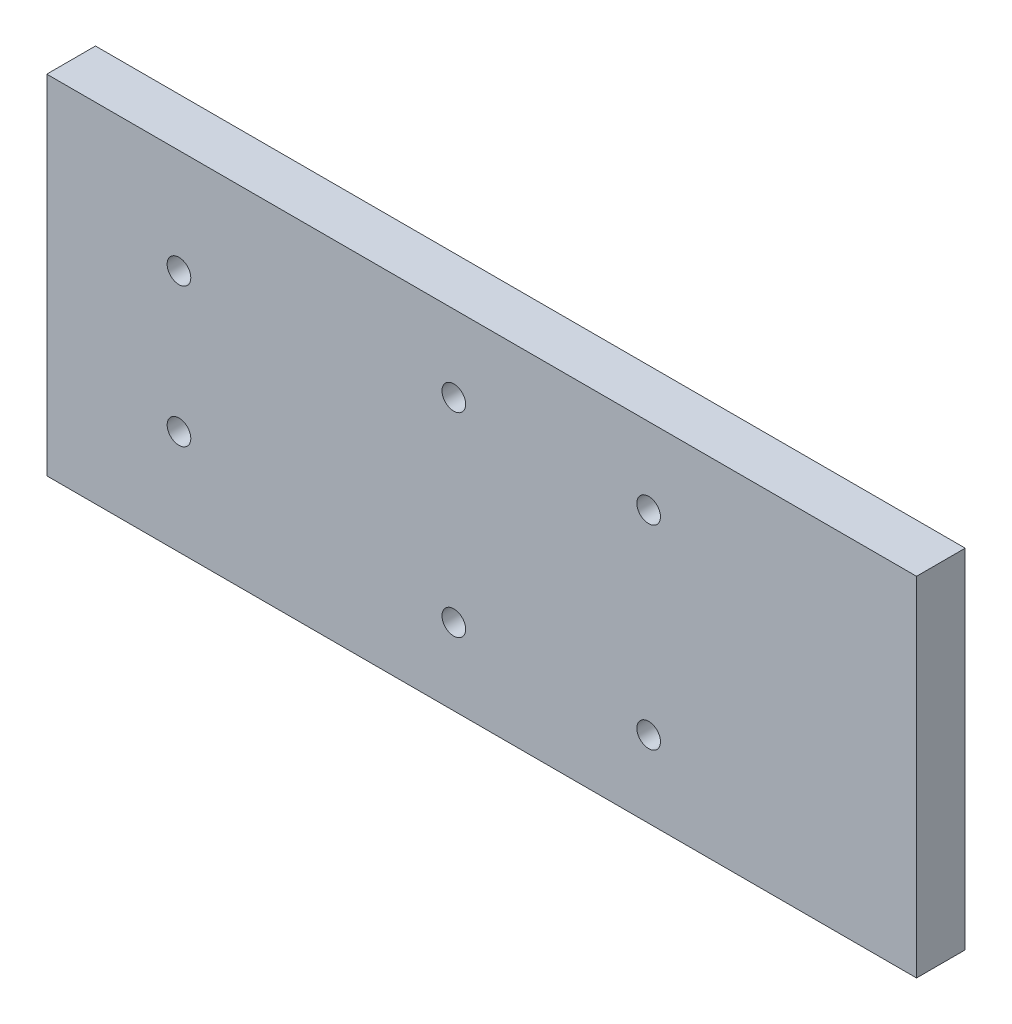
SolidWorks part; units mm, degrees
material "普通碳钢"
ref_plane "Front Plane" through (0, 0, 0) normal (0, 0, 1) x (1, 0, 0)
ref_plane "Top Plane" through (0, 0, 0) normal (0, 1, 0) x (1, 0, 0)
ref_plane "Right Plane" through (0, 0, 0) normal (1, 0, 0) x (0, 0, -1)
sketch "Sketch1" plane through (0, 0, 0) normal (0, 0, 1) x (1, 0, 0)
  line L0 (0, 50) -> (250, 50) construction
  line L1 (0, 0) -> (250, 0)
  line L2 (0, 0) -> (0, 100)
  line L3 (0, 100) -> (250, 100)
  line L4 (250, 0) -> (250, 100)
  line L6 (145, 100) -> (145, 0) construction
  circle A0 centre (117, 78) radius 2.5
  circle A1 centre (173, 78) radius 2.5
  circle A2 centre (117, 22) radius 2.5
  circle A3 centre (173, 22) radius 2.5
  dimension "D4" = 5
  dimension "D1" = 100
  dimension "D2" = 250
  dimension "D3" = 105
  dimension "D5" = 28
  dimension "D6" = 56
  dimension "D7" = 56
  dimension "D8" = 28
extrude "Boss-Extrude1" add sketch "Sketch1" along normal blind 14
hole_wizard "M8 Tapped Hole1" positions "Sketch2" profile "Sketch3" tap size "M8" standard "GB"
sketch "Sketch2" plane through (0, 0, 14) normal (0, 0, 1) x (1, 0, 0)
  point P0 (117, 78)
  point P3 (173, 78)
  point P6 (117, 22)
  point P9 (173, 22)
sketch "Sketch3" plane through (117, 78, 14) normal (1, 0, 0) x (0, -1, 0)
  line L0 (0, 0) -> (0, 21.7929)
  line L1 (0, 21.7929) -> (3.4, 19.75)
  line L2 (3.4, 19.75) -> (3.4, 0)
  line L5 (3.4, 0) -> (0, 0)
  line L10 (0, 21.7929) -> (-3.4, 19.75) construction
  line L11 (0, -6.35) -> (0, 107.95) construction
  dimension "螺纹孔钻头直径" = 6.8
  dimension "螺纹孔钻头深度" = 19.75
  dimension "导头角度" = 118
cosmetic thread "Cosmetic Thread1" parameters "D1"=14, "D2"=8
cosmetic thread "Cosmetic Thread2" parameters "D1"=14, "D2"=8
cosmetic thread "Cosmetic Thread3" parameters "D1"=14, "D2"=8
cosmetic thread "Cosmetic Thread4" parameters "D1"=14, "D2"=8
hole_wizard "M8 Tapped Hole2" positions "Sketch4" profile "Sketch5" tap size "M8" standard "GB" end condition through all
sketch "Sketch4" plane through (0, 0, 14) normal (0, 0, 1) x (1, 0, 0)
  line L0 (0, 50) -> (6.9633, 50) construction
  line L1 (0, 100) -> (0, 0) construction
  point P0 (38, 70)
  point P2 (38, 30)
  dimension "D1" = 40
  dimension "D2" = 38
sketch "Sketch5" plane through (38, 70, 14) normal (1, 0, 0) x (0, -1, 0)
  line L0 (0, 0) -> (0, 14)
  line L1 (0, 14) -> (3.4, 14)
  line L2 (3.4, 14) -> (3.4, 0)
  line L5 (3.4, 0) -> (0, 0)
  line L11 (0, -6.35) -> (0, 107.95) construction
  dimension "通孔螺纹孔钻头直径" = 6.8
  dimension "通孔螺纹孔钻头深度" = 14
cosmetic thread "Cosmetic Thread5" parameters "D2"=8
cosmetic thread "Cosmetic Thread6" parameters "D2"=8
